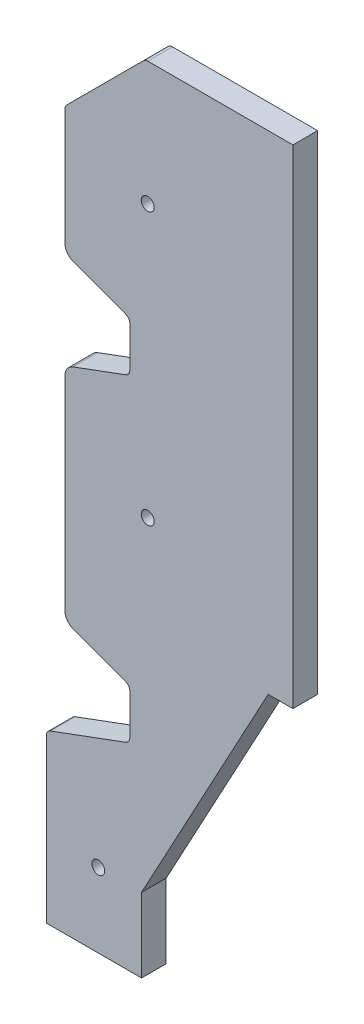
SolidWorks part; units mm, degrees
material "Q235B"
ref_plane "Front Plane" through (0, 0, 0) normal (0, 0, 1) x (1, 0, 0)
ref_plane "Top Plane" through (0, 0, 0) normal (0, 1, 0) x (1, 0, 0)
ref_plane "Right Plane" through (0, 0, 0) normal (1, 0, 0) x (0, 0, -1)
sketch "Sketch1" plane through (0, 0, 0) normal (0, 0, 1) x (1, 0, 0)
  line L0 (154, 0) -> (154, 120)
  line L1 (0, 0) -> (154, 0)
  line L2 (0, 0) -> (0, 1290)
  line L3 (0, 1290) -> (399, 1290)
  line L4 (399, 500) -> (399, 1290)
  line L5 (154, 120) -> (359, 500)
  line L6 (359, 500) -> (399, 500)
  dimension "D1" = 399
  dimension "D2" = 1290
  dimension "D3" = 500
  dimension "D4" = 245
  dimension "D5" = 120
  dimension "D6" = 40
extrude "Boss-Extrude1" add sketch "Sketch1" along normal blind 40
chamfer "Chamfer1" distance 160 angle 45 1 edges at (0, 1290, 20)
hole_wizard "M24 Tapped Hole1" positions "3DSketch1" profile "Sketch2" tap size "M24" standard "GB" end condition up to next
sketch3d "3DSketch1"
  line L0 (399, 1290, 0) -> (160, 1290, 0) construction
  line L1 (399, 500, 0) -> (399, 1290, 0) construction
  line L2 (0, 0, 0) -> (154, 0, 0) construction
  line L3 (154, 0, 0) -> (154, 120, 0) construction
  point P0 (164, 1090, 0)
  point P5 (164, 650, 0)
  point P7 (84, 120, 0)
  dimension "D1" = 200
  dimension "D2" = 235
  dimension "D3" = 235
  dimension "D4" = 650
  dimension "D5" = 70
  dimension "D6" = 120
sketch "Sketch2" plane through (164, 1090, 0) normal (1, 0, 0) x (0, 1, 0)
  line L0 (0, 0) -> (0, 40)
  line L1 (0, 40) -> (10.5, 40)
  line L2 (10.5, 40) -> (10.5, 0)
  line L5 (10.5, 0) -> (0, 0)
  line L11 (0, -6.35) -> (0, 107.95) construction
  dimension "通孔螺纹孔钻头直径" = 21
  dimension "通孔螺纹孔钻头深度" = 40
cosmetic thread "Hole thread 1" parameters "D2"=24
cosmetic thread "Hole thread 2" parameters "D2"=24
cosmetic thread "Hole thread 3" parameters "D2"=24
sketch "Sketch3" plane through (0, 0, 0) normal (0, 0, -1) x (-1, 0, 0)
  line L0 (0, 1130) -> (0, 0) construction
  line L1 (-135, 835) -> (0, 785)
  line L2 (-135, 400) -> (-135, 320)
  line L3 (0, 785) -> (0, 965)
  line L4 (0, 965) -> (-135, 915)
  line L6 (0, 0) -> (-154, 0) construction
  line L7 (-135, 400) -> (0, 450)
  line L8 (-135, 835) -> (-135, 915)
  line L9 (0, 450) -> (0, 270)
  line L10 (0, 270) -> (-135, 320)
  dimension "D1" = 320
  dimension "D2" = 435
  dimension "D3" = 135
  dimension "D4" = 80
  dimension "D5" = 80
  dimension "D6" = 180
  dimension "D7" = 135
  dimension "D8" = 180
  dimension "D9" = 50
extrude "Cut-Extrude1" cut sketch "Sketch3" against normal through all
fillet "Fillet1" radius 10 8 edges at (135, 835, 20) (135, 915, 20) (0, 965, 20) (0, 785, 20) (0, 270, 20) (0, 450, 20) (135, 400, 20) (135, 320, 20)
sketch "Sketch4" plane through (0, 0, 0) normal (0, 0, -1) x (-1, 0, 0)
  line L0 (0, 1130) -> (-160, 1290) construction
  line L1 (0, 337.1812) -> (-30, 337.1812)
  line L2 (0, 337.1812) -> (0, 1160)
  line L3 (0, 1160) -> (-30, 1160)
  line L4 (-30, 337.1812) -> (-30, 1160)
  line L5 (0, 1130) -> (0, 971.9601) construction
  dimension "D1" = 30
extrude "Cut-Extrude2" cut sketch "Sketch4" against normal through all
fillet "Fillet2" radius 20 3 edges at (30, 438.8889, 20) (30, 796.1111, 20) (30, 953.8889, 20)
fillet "Fillet3" radius 10 2 edges at (160, 1290, 20) (30, 1160, 20)
